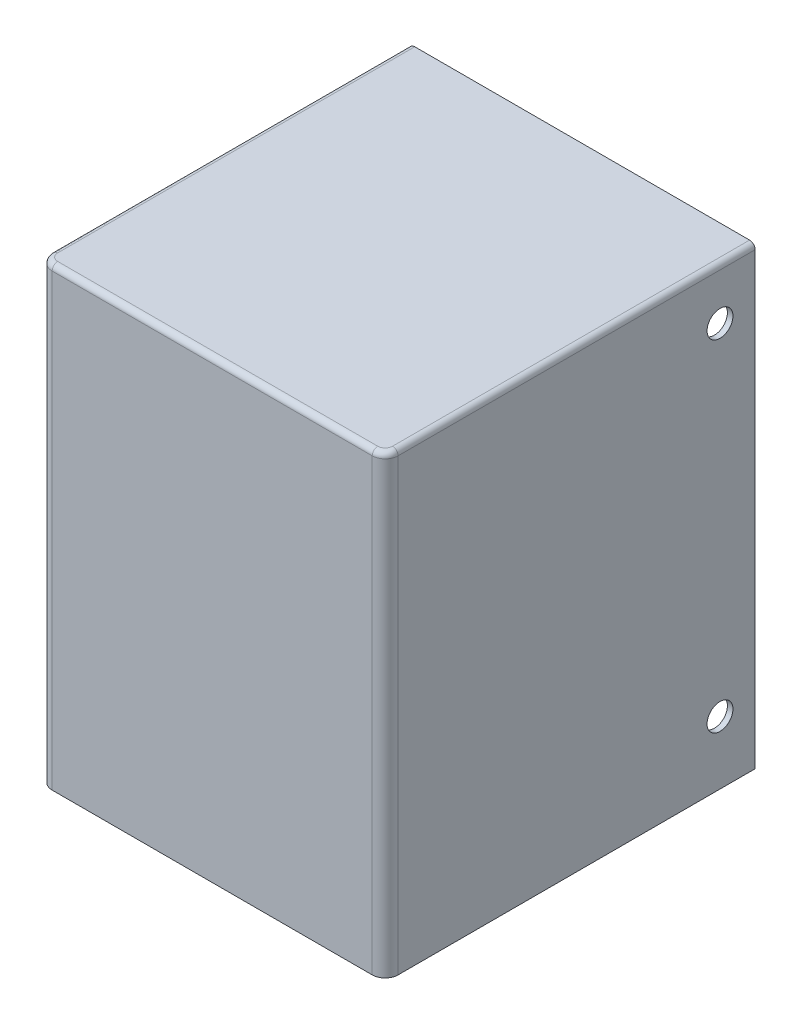
SolidWorks part; units mm, degrees
material "SUS304"
ref_plane "前视基准面" through (0, 0, 0) normal (0, 0, 1) x (1, 0, 0)
ref_plane "上视基准面" through (0, 0, 0) normal (0, 1, 0) x (1, 0, 0)
ref_plane "右视基准面" through (0, 0, 0) normal (1, 0, 0) x (0, 0, -1)
sketch "草图1" plane through (0, 0, 0) normal (0, 0, 1) x (1, 0, 0)
  line L1 (-45.25, 60) -> (45.25, 60)
  line L2 (-45.25, 60) -> (-45.25, -60)
  line L3 (-45.25, -60) -> (45.25, -60)
  line L4 (45.25, 60) -> (45.25, -60)
  line L5 (-45.25, 60) -> (45.25, -60) construction
  line L6 (-45.25, -60) -> (45.25, 60) construction
  line L7 (-46.75, 61.5) -> (46.75, 61.5)
  line L8 (-46.75, 61.5) -> (-46.75, -61.5)
  line L9 (-46.75, -61.5) -> (46.75, -61.5)
  line L10 (46.75, 61.5) -> (46.75, -61.5)
  line L11 (-46.75, 61.5) -> (46.75, -61.5) construction
  line L12 (-46.75, -61.5) -> (46.75, 61.5) construction
  point P0 (0, 0)
  point P6 (0, 0)
  dimension "D1" = 90.5
  dimension "D2" = 120
  dimension "D3" = 1.5
  dimension "D4" = 1.5
extrude "凸台-拉伸1" add sketch "草图1" along normal blind 100
sketch "草图2" plane through (0, 0, 100) normal (0, 0, 1) x (1, 0, 0)
  line L1 (-46.75, 61.5) -> (46.75, 61.5)
  line L2 (-46.75, 61.5) -> (-46.75, -61.5)
  line L3 (-46.75, -61.5) -> (46.75, -61.5)
  line L4 (46.75, 61.5) -> (46.75, -61.5)
  line L5 (-46.75, 61.5) -> (46.75, -61.5) construction
  line L6 (-46.75, -61.5) -> (46.75, 61.5) construction
  point P0 (0, 0)
extrude "凸台-拉伸2" add sketch "草图2" against normal blind 1.5
sketch "草图3" plane through (0, -61.5, 0) normal (0, -1, 0) x (1, 0, 0)
  line L1 (-45.25, 0) -> (45.25, 0)
  line L2 (-45.25, 0) -> (-45.25, 98.5)
  line L3 (-45.25, 98.5) -> (45.25, 98.5)
  line L4 (45.25, 0) -> (45.25, 98.5)
extrude "切除-拉伸1" cut sketch "草图3" against normal blind 3
sketch "草图4" plane through (46.75, 0, 0) normal (1, 0, 0) x (0, 0, -1)
  line L0 (0, -61.5) -> (0, 61.5) construction
  line L3 (-18.5, 57.5) -> (-0.5, 57.5) construction
  circle A0 centre (-9.5, -44.5) radius 3.5
  circle A1 centre (-9.5, 47.5) radius 3.5
  dimension "D1" = 7
  dimension "D2" = 9.5
  dimension "D3" = 7
  dimension "D4" = 10
  dimension "D5" = 9.5
  dimension "D6" = 92
extrude "切除-拉伸2" cut sketch "草图4" against normal through all
fillet "圆角1" radius 2 2 edges at (-45.25, -0.75, 98.5) (45.25, -0.75, 98.5)
fillet "圆角2" radius 3.5 2 edges at (46.75, 0, 100) (-46.75, 0, 100)
fillet "圆角3" radius 1 5 edges at (45.25, 60, 48.25) (44.6642, 60, 97.9142) (-45.25, 60, 48.25) (-44.6642, 60, 97.9142) (0, 60, 98.5)
fillet "圆角4" radius 1.5 5 edges at (46.75, 61.5, 48.25) (45.7249, 61.5, 98.9749) (-46.75, 61.5, 48.25) (-45.7249, 61.5, 98.9749) (0, 61.5, 100)
